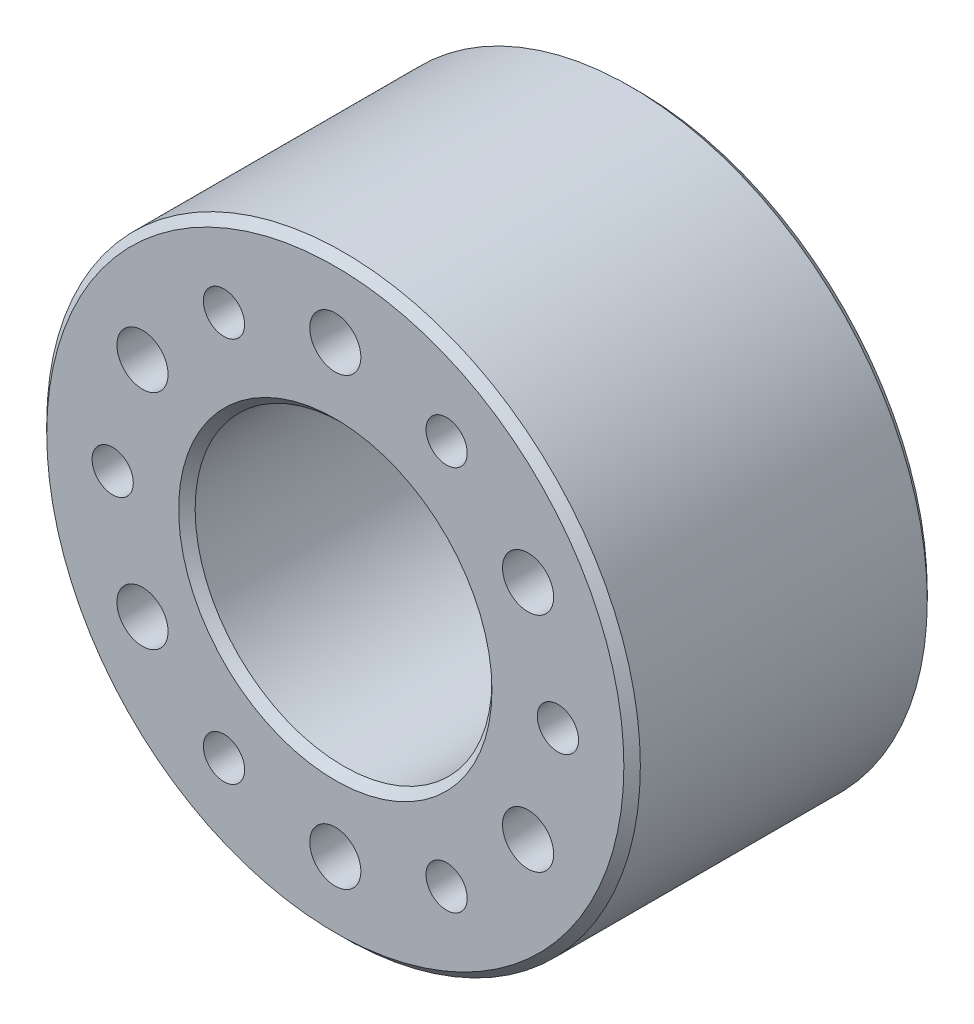
from build123d import *

# Parameters (mm, degrees)
SKETCH_1_R          = 18
SKETCH_1_R_2        = 1.55
SKETCH_1_R_3        = 9
EXTRUDE_1_DEPTH     = 18.4
SKETCH_4_R          = 3.5
CUT_EXTRUDE_1_DEPTH = 7
EXTRUDE_START       = 4
SKETCH_5_R          = 10
SKETCH_5_R_2        = 9
EXTRUDE_2_DEPTH     = 4
HOLE_WIZARD_M3_1_D  = 2.5
CHAMFER_1_SIZE      = 0.5


with BuildPart() as part:
    # 草图1 → 凸台-拉伸1 (new body)
    with BuildSketch(Plane.XY):
        with Locations(Location((0, 0, 0), (0, 0, 180))):
            Circle(SKETCH_1_R)
        with Locations(Location((0, 13.5, 0), (0, 0, 180))):
            Circle(SKETCH_1_R_2, mode=Mode.SUBTRACT)
        with Locations(Location((11.691342951, 6.75, 0), (0, 0, 180))):
            Circle(SKETCH_1_R_2, mode=Mode.SUBTRACT)
        with Locations(Location((11.691342951, -6.75, 0), (0, 0, 180))):
            Circle(SKETCH_1_R_2, mode=Mode.SUBTRACT)
        with Locations(Location((0, -13.5, 0), (0, 0, 180))):
            Circle(SKETCH_1_R_2, mode=Mode.SUBTRACT)
        with Locations(Location((-11.691342951, -6.75, 0), (0, 0, 180))):
            Circle(SKETCH_1_R_2, mode=Mode.SUBTRACT)
        with Locations(Location((-11.691342951, 6.75, 0), (0, 0, 180))):
            Circle(SKETCH_1_R_2, mode=Mode.SUBTRACT)
        with Locations(Location((0, 0, 0), (0, 0, 180))):
            Circle(SKETCH_1_R_3, mode=Mode.SUBTRACT)
    extrude(amount=EXTRUDE_1_DEPTH)

    # 草图4 → 切除-拉伸1 (cut)
    with BuildSketch(Plane.XY):
        with Locations((0, 13.5)):
            Circle(SKETCH_4_R)
        with Locations((11.691342951, 6.75)):
            Circle(SKETCH_4_R)
        with Locations((11.691342951, -6.75)):
            Circle(SKETCH_4_R)
        with Locations((0, -13.5)):
            Circle(SKETCH_4_R)
        with Locations((-11.691342951, -6.75)):
            Circle(SKETCH_4_R)
        with Locations((-11.691342951, 6.75)):
            Circle(SKETCH_4_R)
    extrude(amount=CUT_EXTRUDE_1_DEPTH, mode=Mode.SUBTRACT)

    # 草图5 → 凸台-拉伸2 (add)
    with BuildSketch(Plane(origin=(0, 0, 0), x_dir=(-1, 0, 0), z_dir=(0, 0, -1)).offset(EXTRUDE_START)):
        with Locations(Location((0, 0, 0), (0, 0, 209.999869527))):
            Circle(SKETCH_5_R)
        Circle(SKETCH_5_R_2, mode=Mode.SUBTRACT)
    extrude(amount=-EXTRUDE_2_DEPTH)

    # M3 螺纹孔1 (through all)
    with Locations(Plane.XY.offset(18.4)):
        with Locations((13.5, 0), (6.75, -11.691342951), (-6.75, -11.691342951), (-13.5, 0), (-6.75, 11.691342951), (6.75, 11.691342951)):
            Hole(HOLE_WIZARD_M3_1_D / 2)

    # 倒角1
    chamfer_1_edges = [part.edges().sort_by_distance(p)[0] for p in [
        (18, 0, 0),
        (9, 0, 18.4),
        (18, 0, 18.4),
        (-8.660265424, 4.999980279, -4),
    ]]
    chamfer(chamfer_1_edges, length=CHAMFER_1_SIZE)


solid = part.part
